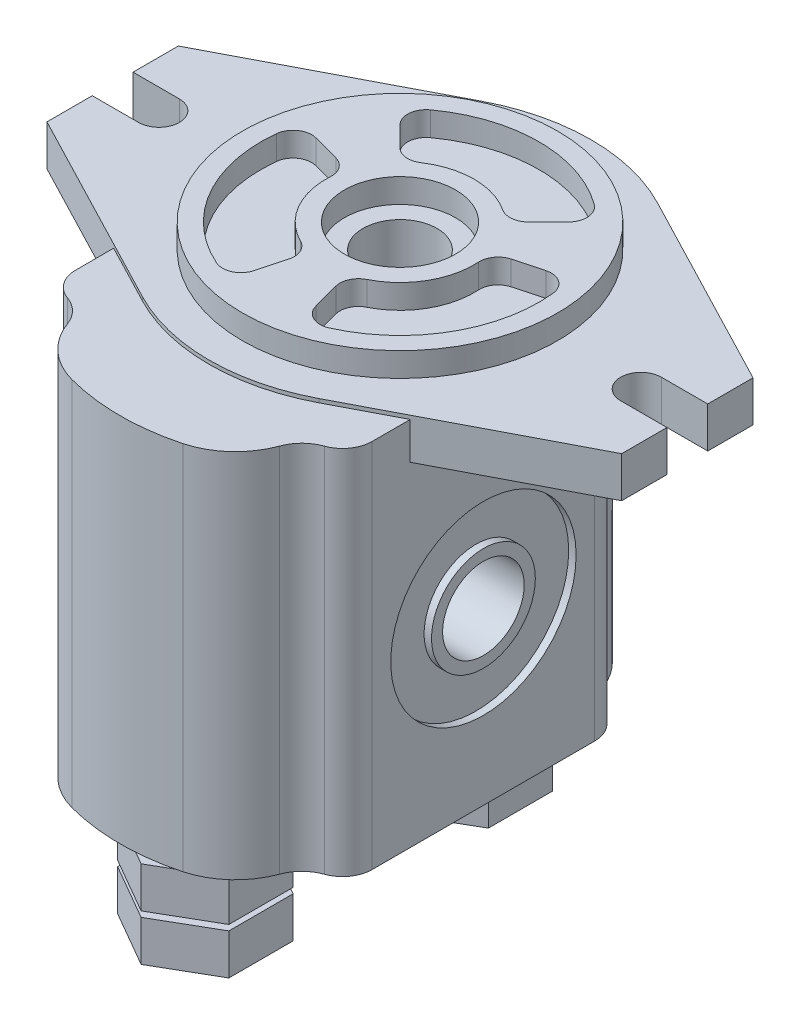
SolidWorks part; units mm, degrees
ref_plane "Front Plane" through (0, 0, 0) normal (0, 0, 1) x (1, 0, 0)
ref_plane "Top Plane" through (0, 0, 0) normal (0, 1, 0) x (1, 0, 0)
ref_plane "Right Plane" through (0, 0, 0) normal (1, 0, 0) x (0, 0, -1)
sketch "Sketch 1" plane through (0, 0, 0) normal (0, 1, 0) x (1, 0, 0)
  line L0 (0, 73.1544) -> (0, -87.1141) construction
  line L1 (-89.396, 0) -> (95.5705, 0) construction
  line L2 (-40, 30) -> (-40, -30)
  line L3 (40, 30) -> (40, -30)
  arc A0 (14.9706, 56.0346) -> (-14.9706, 56.0346) centre (0, 0) ccw
  arc A1 (-34.6667, 37.5425) -> (-28.6028, 43.5512) centre (-38, 46.9706) ccw
  arc A2 (-34.6667, 37.5425) -> (-40, 30) centre (-32, 30) ccw
  arc A3 (-14.9706, 56.0346) -> (-28.6028, 43.5512) centre (-9.8084, 36.7123) ccw
  arc A4 (-14.9706, -56.0346) -> (-28.6028, -43.5512) centre (-9.8084, -36.7123) cw
  arc A5 (-34.6667, -37.5425) -> (-40, -30) centre (-32, -30) cw
  arc A6 (-34.6667, -37.5425) -> (-28.6028, -43.5512) centre (-38, -46.9706) cw
  arc A7 (14.9706, -56.0346) -> (-14.9706, -56.0346) centre (0, 0) cw
  arc A8 (34.6667, -37.5425) -> (28.6028, -43.5512) centre (38, -46.9706) ccw
  arc A9 (34.6667, -37.5425) -> (40, -30) centre (32, -30) ccw
  arc A10 (14.9706, -56.0346) -> (28.6028, -43.5512) centre (9.8084, -36.7123) ccw
  arc A11 (14.9706, 56.0346) -> (28.6028, 43.5512) centre (9.8084, 36.7123) cw
  arc A12 (34.6667, 37.5425) -> (40, 30) centre (32, 30) cw
  arc A13 (34.6667, 37.5425) -> (28.6028, 43.5512) centre (38, 46.9706) cw
  circle A14 centre (0, 17.5) radius 42.5 construction
  point P7 (40, 0)
  point P23 (-40, 0)
  point P38 (0, 60)
  point P41 (0, 58)
  dimension "D2" = 20
  dimension "D4" = 17.5
  dimension "D5" = 85
  dimension "D7" = 10
  dimension "D8" = 8
  dimension "D1" = 80
  dimension "D3" = 60
  dimension "D6" = 2
  dimension "D9" = 38
extrude "Boss-Extrude 1" add sketch "Sketch 1" along normal blind 100
sketch "Sketch 2" plane through (0, 100, 0) normal (0, 1, 0) x (1, 0, 0)
  line L0 (0, 82.4306) -> (0, -30.4305) construction
  line L1 (-109.1302, 17.5) -> (97.471, 17.5) construction
  line L2 (-23.7801, 63.1811) -> (-77.5, 35.2162)
  line L3 (-77.5, 35.2162) -> (-77.5, 23)
  line L4 (-65, 23) -> (-77.5, 23)
  line L5 (-65, 12) -> (-77.5, 12)
  line L6 (-77.5, -0.2162) -> (-77.5, 12)
  line L7 (-23.7801, -28.1811) -> (-77.5, -0.2162)
  line L8 (23.7801, -28.1811) -> (77.5, -0.2162)
  line L9 (77.5, -0.2162) -> (77.5, 12)
  line L10 (65, 12) -> (77.5, 12)
  line L11 (65, 23) -> (77.5, 23)
  line L12 (77.5, 35.2162) -> (77.5, 23)
  line L13 (23.7801, 63.1811) -> (77.5, 35.2162)
  arc A0 (23.7801, 63.1811) -> (-23.7801, 63.1811) centre (0, 17.5) ccw
  arc A1 (-14.9706, -56.0346) -> (14.9706, -56.0346) centre (0, 0) ccw construction
  arc A2 (-65, 12) -> (-65, 23) centre (-65, 17.5) ccw
  arc A3 (23.7801, -28.1811) -> (-23.7801, -28.1811) centre (0, 17.5) cw
  arc A4 (65, 12) -> (65, 23) centre (65, 17.5) cw
  point P6 (0, 69)
  point P7 (0, -58)
  point P23 (0, -34)
  dimension "D2" = 130
  dimension "D1" = 127
  dimension "D3" = 155
  dimension "D4" = 11
  dimension "D5" = 125
extrude "Boss-Extrude 2" add sketch "Sketch 2" along normal blind 1 and the other way blind 10
sketch "Sketch 3" plane through (0, 101, 0) normal (0, 1, 0) x (1, 0, 0)
  line L0 (-22.7074, 40.2074) -> (-17.3205, 34.8205)
  line L1 (0, 71.0981) -> (0, -41.0552) construction
  line L2 (0, 73.1544) -> (0, -87.1141) construction
  line L3 (22.7074, 40.2074) -> (17.3205, 34.8205)
  line L4 (31.0189, 25.8115) -> (23.6603, 23.8397)
  line L5 (8.3115, -13.5189) -> (6.3397, -6.1603)
  line L6 (-8.3115, -13.5189) -> (-6.3397, -6.1603)
  line L7 (-31.0189, 25.8115) -> (-23.6603, 23.8397)
  circle A0 centre (0, 17.5) radius 42.5 construction
  circle A1 centre (0, 17.5) radius 42.5
  circle A2 centre (0, 17.5) radius 15
  arc A3 (22.1214, 47.7803) -> (-22.1214, 47.7803) centre (0, 17.5) ccw
  arc A4 (11.028, 34.1848) -> (-11.028, 34.1848) centre (0, 17.5) ccw
  arc A5 (17.3205, 34.8205) -> (11.028, 34.1848) centre (13.785, 38.356) cw
  arc A6 (22.1214, 47.7803) -> (22.7074, 40.2074) centre (19.1718, 43.7429) cw
  arc A7 (-22.7074, 40.2074) -> (-22.1214, 47.7803) centre (-19.1718, 43.7429) cw
  arc A8 (-11.028, 34.1848) -> (-17.3205, 34.8205) centre (-13.785, 38.356) cw
  arc A9 (15.1628, -16.7978) -> (37.2842, 21.5175) centre (0, 17.5) ccw
  arc A10 (31.0189, 25.8115) -> (37.2842, 21.5175) centre (32.3129, 20.9818) cw
  arc A11 (19.9635, 18.7081) -> (23.6603, 23.8397) centre (24.9543, 19.0101) cw
  arc A12 (8.9355, -0.3929) -> (19.9635, 18.7081) centre (0, 17.5) ccw
  arc A13 (6.3397, -6.1603) -> (8.9355, -0.3929) centre (11.1694, -4.8662) cw
  arc A14 (15.1628, -16.7978) -> (8.3115, -13.5189) centre (13.1411, -12.2248) cw
  arc A15 (-37.2842, 21.5175) -> (-15.1628, -16.7978) centre (0, 17.5) ccw
  arc A16 (-8.3115, -13.5189) -> (-15.1628, -16.7978) centre (-13.1411, -12.2248) cw
  arc A17 (-8.9355, -0.3929) -> (-6.3397, -6.1603) centre (-11.1694, -4.8662) cw
  arc A18 (-19.9635, 18.7081) -> (-8.9355, -0.3929) centre (0, 17.5) ccw
  arc A19 (-23.6603, 23.8397) -> (-19.9635, 18.7081) centre (-24.9543, 19.0101) cw
  arc A20 (-37.2842, 21.5175) -> (-31.0189, 25.8115) centre (-32.3129, 20.9818) cw
  point P47 (0, 17.5)
  dimension "D1" = 30
  dimension "D3" = 5
  dimension "D4" = 5
  dimension "D5" = 5
  dimension "D2" = 90
  dimension "D6" = 3
extrude "Boss-Extrude 3" add sketch "Sketch 3" along normal blind 6.5
sketch "Sketch 4" plane through (0, 101, 0) normal (0, 1, 0) x (1, 0, 0)
  circle A0 centre (0, 17.5) radius 10
  dimension "D1" = 20
extrude "Cut-Extrude 1" cut sketch "Sketch 4" against normal blind 50
sketch "Sketch 5" plane through (0, 0, 0) normal (0, -1, 0) x (1, 0, 0)
  line L0 (49.0169, 0) -> (-44.4216, 0) construction
  line L1 (0, -78.1318) -> (0, 88.0661) construction
  circle A0 centre (0, -35) radius 11
  circle A1 centre (0, 35) radius 11
  dimension "D1" = 22
  dimension "D2" = 70
extrude "Boss-Extrude 4" add sketch "Sketch 5" along normal blind 20
sketch "Sketch 6" plane through (40, 0, 0) normal (1, 0, 0) x (0, 0, -1)
  line L0 (0, 127.4556) -> (0, -15.0849) construction
  line L1 (60, 101) -> (-25, 101) construction
  circle A0 centre (0, 46) radius 25
  circle A1 centre (0, 46) radius 14
  dimension "D1" = 50
  dimension "D3" = 28
  dimension "D2" = 55
extrude "Cut-Extrude 2" cut sketch "Sketch 6" against normal blind 2
sketch "Sketch 7" plane through (40, 0, 0) normal (1, 0, 0) x (0, 0, -1)
  circle A0 centre (0, 46) radius 11
  dimension "D1" = 22
extrude "Cut-Extrude 3" cut sketch "Sketch 7" against normal blind 20
mirror "Mirror 1" about plane through (0, 0, 0) normal (1, 0, 0) of "Cut-Extrude 3", "Cut-Extrude 2"
sketch "Sketch 9" plane through (0, -20, 0) normal (0, -1, 0) x (1, 0, 0)
  line L0 (47.4785, 0) -> (-51.0531, 0) construction
  line L1 (0, -52.3205) -> (15, -43.6603)
  line L2 (15, -43.6603) -> (15, -26.3397)
  line L3 (15, -26.3397) -> (0, -17.6795)
  line L4 (0, -17.6795) -> (-15, -26.3397)
  line L5 (-15, -26.3397) -> (-15, -43.6603)
  line L6 (-15, -43.6603) -> (0, -52.3205)
  line L7 (-15, 43.6603) -> (0, 52.3205)
  line L8 (-15, 26.3397) -> (-15, 43.6603)
  line L9 (0, 17.6795) -> (-15, 26.3397)
  line L10 (15, 26.3397) -> (0, 17.6795)
  line L11 (15, 43.6603) -> (15, 26.3397)
  line L12 (0, 52.3205) -> (15, 43.6603)
  circle A0 centre (0, -35) radius 15 construction
  circle A1 centre (0, 35) radius 15 construction
  dimension "D1" = 30
extrude "Boss-Extrude 5" add sketch "Sketch 9" against normal blind 11 from offset 1.5 offset against normal yes
sketch "Sketch 10" plane through (0, -20, 0) normal (0, -1, 0) x (1, 0, 0)
  line L0 (-15, 43.6603) -> (-15, 26.3397) construction
  line L1 (-15, 26.3397) -> (0, 17.6795) construction
  line L2 (0, 17.6795) -> (15, 26.3397) construction
  line L3 (15, 26.3397) -> (15, 43.6603) construction
  line L4 (15, 43.6603) -> (0, 52.3205) construction
  line L5 (0, 52.3205) -> (-15, 43.6603) construction
  line L6 (-15, -43.6603) -> (0, -52.3205) construction
  line L7 (0, -52.3205) -> (15, -43.6603) construction
  line L8 (15, -43.6603) -> (15, -26.3397) construction
  line L9 (15, -26.3397) -> (0, -17.6795) construction
  line L10 (0, -17.6795) -> (-15, -26.3397) construction
  line L11 (-15, -26.3397) -> (-15, -43.6603) construction
  line L12 (-15, 43.6603) -> (-15, 26.3397)
  line L13 (-15, 26.3397) -> (0, 17.6795)
  line L14 (0, 17.6795) -> (15, 26.3397)
  line L15 (15, 26.3397) -> (15, 43.6603)
  line L16 (15, 43.6603) -> (0, 52.3205)
  line L17 (0, 52.3205) -> (-15, 43.6603)
  line L18 (-15, -43.6603) -> (0, -52.3205)
  line L19 (0, -52.3205) -> (15, -43.6603)
  line L20 (15, -43.6603) -> (15, -26.3397)
  line L21 (15, -26.3397) -> (0, -17.6795)
  line L22 (0, -17.6795) -> (-15, -26.3397)
  line L23 (-15, -26.3397) -> (-15, -43.6603)
extrude "Boss-Extrude 6" add sketch "Sketch 10" along normal blind 11
sketch "Sketch 11" plane through (0, -31, 0) normal (0, -1, 0) x (1, 0, 0)
  line L0 (27.2316, 0) -> (-33.614, 0) construction
  line L1 (15, -35) -> (-15, -35) construction
  line L2 (15, -43.6603) -> (15, -26.3397) construction
  line L3 (-15, -26.3397) -> (-15, -43.6603) construction
  line L4 (15, 35) -> (-15, 35) construction
  circle A0 centre (0, -35) radius 11
  circle A1 centre (0, 35) radius 11
  dimension "D1" = 22
extrude "Cut-Extrude 4" cut sketch "Sketch 11" against normal blind 6
